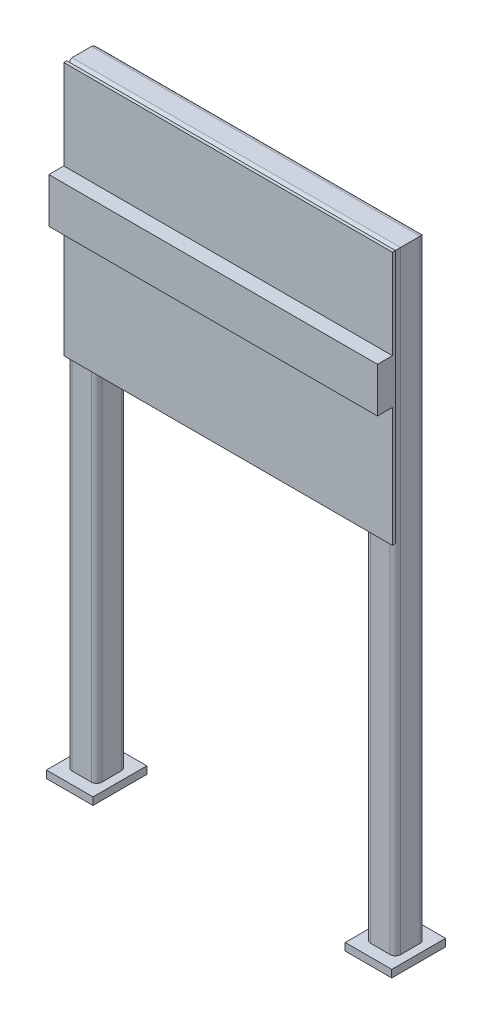
from build123d import *

# Parameters (mm, degrees)
GB_6728_1986_SQUARE_HOLLOW_SECTION_020_X_DEPTH = 415.142135624
GB_6728_1986_SQUARE_HOLLOW_SECTION_0_3_DEPTH   = 230.284271247
GB_6728_1986_SQUARE_HOLLOW_SECTION_0_5_DEPTH   = 415.142135624
GB_6728_1986_SQUARE_HOLLOW_SECTION_0_6_DEPTH   = 202
GB_6728_1986_SQUARE_HOLLOW_SECTION_0_8_DEPTH   = 202
SKETCH2_W                                      = 31.17404588
SKETCH2_H                                      = 36.03704403
BOSS_EXTRUDE1_DEPTH                            = 5
SKETCH3_W                                      = 220
SKETCH3_H                                      = 170
BOSS_EXTRUDE2_DEPTH                            = 2
SKETCH4_W                                      = 220
SKETCH4_H                                      = 30
BOSS_EXTRUDE3_DEPTH                            = 10


with BuildPart() as part:
    # Sketch1 → GB/6728-1986 square hollow section 020 X 20 X 1.75(1) (new body)
    with BuildSketch(Plane(origin=(-100, 0, 0), x_dir=(-1, 0, 0), z_dir=(0, 1, 0))):
        with BuildLine():
            Line((-6.5, -10), (6.5, -10))
            ThreePointArc((6.5, -10), (8.974873734, -8.974873734), (10, -6.5))
            Line((10, -6.5), (10, 6.5))
            ThreePointArc((10, 6.5), (8.974873734, 8.974873734), (6.5, 10))
            Line((6.5, 10), (-6.5, 10))
            ThreePointArc((-6.5, 10), (-8.974873734, 8.974873734), (-10, 6.5))
            Line((-10, 6.5), (-10, -6.5))
            ThreePointArc((-10, -6.5), (-8.974873734, -8.974873734), (-6.5, -10))
        make_face()
        with BuildLine():
            Line((-6.5, -8.25), (6.5, -8.25))
            ThreePointArc((6.5, -8.25), (7.737436867, -7.737436867), (8.25, -6.5))
            Line((8.25, -6.5), (8.25, 6.5))
            ThreePointArc((8.25, 6.5), (7.737436867, 7.737436867), (6.5, 8.25))
            Line((6.5, 8.25), (-6.5, 8.25))
            ThreePointArc((-6.5, 8.25), (-7.737436867, 7.737436867), (-8.25, 6.5))
            Line((-8.25, 6.5), (-8.25, -6.5))
            ThreePointArc((-8.25, -6.5), (-7.737436867, -7.737436867), (-6.5, -8.25))
        make_face(mode=Mode.SUBTRACT)
    extrude(amount=GB_6728_1986_SQUARE_HOLLOW_SECTION_020_X_DEPTH)

    # GB_6728-1986 square hollow section 0 2
    split(bisect_by=Plane(origin=(-100, 400, 0), x_dir=(0.707106781, -0.707106781, 0), z_dir=(-0.707106781, -0.707106781, 0)), keep=Keep.TOP)



with BuildPart() as body_2:
    # Sketch1 on segment 2 (carried to segment 2) → GB_6728-1986 square hollow section 0 3 (new body)
    with BuildSketch(Plane(origin=(-115.142135624, 400, 0), x_dir=(0, 1, 0), z_dir=(1, 0, 0))):
        with BuildLine():
            Line((-6.5, -10), (6.5, -10))
            ThreePointArc((6.5, -10), (8.974873734, -8.974873734), (10, -6.5))
            Line((10, -6.5), (10, 6.5))
            ThreePointArc((10, 6.5), (8.974873734, 8.974873734), (6.5, 10))
            Line((6.5, 10), (-6.5, 10))
            ThreePointArc((-6.5, 10), (-8.974873734, 8.974873734), (-10, 6.5))
            Line((-10, 6.5), (-10, -6.5))
            ThreePointArc((-10, -6.5), (-8.974873734, -8.974873734), (-6.5, -10))
        make_face()
        with BuildLine():
            Line((-6.5, -8.25), (6.5, -8.25))
            ThreePointArc((6.5, -8.25), (7.737436867, -7.737436867), (8.25, -6.5))
            Line((8.25, -6.5), (8.25, 6.5))
            ThreePointArc((8.25, 6.5), (7.737436867, 7.737436867), (6.5, 8.25))
            Line((6.5, 8.25), (-6.5, 8.25))
            ThreePointArc((-6.5, 8.25), (-7.737436867, 7.737436867), (-8.25, 6.5))
            Line((-8.25, 6.5), (-8.25, -6.5))
            ThreePointArc((-8.25, -6.5), (-7.737436867, -7.737436867), (-6.5, -8.25))
        make_face(mode=Mode.SUBTRACT)
    extrude(amount=GB_6728_1986_SQUARE_HOLLOW_SECTION_0_3_DEPTH)

    # GB_6728-1986 square hollow section 0 3 m
    split(bisect_by=Plane(origin=(-100, 400, 0), x_dir=(-0.707106781, 0.707106781, 0), z_dir=(0.707106781, 0.707106781, 0)), keep=Keep.TOP)

    # GB_6728-1986 square hollow section 0 4
    split(bisect_by=Plane(origin=(100, 400, 0), x_dir=(-0.707106781, -0.707106781, 0), z_dir=(-0.707106781, 0.707106781, 0)), keep=Keep.TOP)


with BuildPart() as body_3:
    # Sketch1 on segment 3 (carried to segment 3) → GB_6728-1986 square hollow section 0 5 (new body)
    with BuildSketch(Plane(origin=(100, 415.142135624, 0), x_dir=(1, 0, 0), z_dir=(0, -1, 0))):
        with BuildLine():
            Line((-6.5, -10), (6.5, -10))
            ThreePointArc((6.5, -10), (8.974873734, -8.974873734), (10, -6.5))
            Line((10, -6.5), (10, 6.5))
            ThreePointArc((10, 6.5), (8.974873734, 8.974873734), (6.5, 10))
            Line((6.5, 10), (-6.5, 10))
            ThreePointArc((-6.5, 10), (-8.974873734, 8.974873734), (-10, 6.5))
            Line((-10, 6.5), (-10, -6.5))
            ThreePointArc((-10, -6.5), (-8.974873734, -8.974873734), (-6.5, -10))
        make_face()
        with BuildLine():
            Line((-6.5, -8.25), (6.5, -8.25))
            ThreePointArc((6.5, -8.25), (7.737436867, -7.737436867), (8.25, -6.5))
            Line((8.25, -6.5), (8.25, 6.5))
            ThreePointArc((8.25, 6.5), (7.737436867, 7.737436867), (6.5, 8.25))
            Line((6.5, 8.25), (-6.5, 8.25))
            ThreePointArc((-6.5, 8.25), (-7.737436867, 7.737436867), (-8.25, 6.5))
            Line((-8.25, 6.5), (-8.25, -6.5))
            ThreePointArc((-8.25, -6.5), (-7.737436867, -7.737436867), (-6.5, -8.25))
        make_face(mode=Mode.SUBTRACT)
    extrude(amount=GB_6728_1986_SQUARE_HOLLOW_SECTION_0_5_DEPTH)

    # GB_6728-1986 square hollow section 0 5 m
    split(bisect_by=Plane(origin=(100, 400, 0), x_dir=(0.707106781, 0.707106781, 0), z_dir=(0.707106781, -0.707106781, 0)), keep=Keep.TOP)


with BuildPart() as body_4:
    # Sketch1 on segment 4 (carried to segment 4) → GB_6728-1986 square hollow section 0 6 (new body)
    with BuildSketch(Plane(origin=(-101, 330, 0), x_dir=(0, 1, 0), z_dir=(1, 0, 0))):
        with BuildLine():
            Line((-6.5, -10), (6.5, -10))
            ThreePointArc((6.5, -10), (8.974873734, -8.974873734), (10, -6.5))
            Line((10, -6.5), (10, 6.5))
            ThreePointArc((10, 6.5), (8.974873734, 8.974873734), (6.5, 10))
            Line((6.5, 10), (-6.5, 10))
            ThreePointArc((-6.5, 10), (-8.974873734, 8.974873734), (-10, 6.5))
            Line((-10, 6.5), (-10, -6.5))
            ThreePointArc((-10, -6.5), (-8.974873734, -8.974873734), (-6.5, -10))
        make_face()
        with BuildLine():
            Line((-6.5, -8.25), (6.5, -8.25))
            ThreePointArc((6.5, -8.25), (7.737436867, -7.737436867), (8.25, -6.5))
            Line((8.25, -6.5), (8.25, 6.5))
            ThreePointArc((8.25, 6.5), (7.737436867, 7.737436867), (6.5, 8.25))
            Line((6.5, 8.25), (-6.5, 8.25))
            ThreePointArc((-6.5, 8.25), (-7.737436867, 7.737436867), (-8.25, 6.5))
            Line((-8.25, 6.5), (-8.25, -6.5))
            ThreePointArc((-8.25, -6.5), (-7.737436867, -7.737436867), (-6.5, -8.25))
        make_face(mode=Mode.SUBTRACT)
    extrude(amount=GB_6728_1986_SQUARE_HOLLOW_SECTION_0_6_DEPTH)

    # GB_6728-1986 square hollow section 0 6 m
    split(bisect_by=Plane(origin=(-90, 330, 0), x_dir=(0, 1, 0), z_dir=(1, 0, 0)), keep=Keep.TOP)

    # GB_6728-1986 square hollow section 0 7
    split(bisect_by=Plane(origin=(90, 330, 0), x_dir=(0, -1, 0), z_dir=(-1, 0, 0)), keep=Keep.TOP)


with BuildPart() as body_5:
    # Sketch1 on segment 5 (carried to segment 5) → GB_6728-1986 square hollow section 0 8 (new body)
    with BuildSketch(Plane(origin=(-101, 250, 0), x_dir=(0, 1, 0), z_dir=(1, 0, 0))):
        with BuildLine():
            Line((-6.5, -10), (6.5, -10))
            ThreePointArc((6.5, -10), (8.974873734, -8.974873734), (10, -6.5))
            Line((10, -6.5), (10, 6.5))
            ThreePointArc((10, 6.5), (8.974873734, 8.974873734), (6.5, 10))
            Line((6.5, 10), (-6.5, 10))
            ThreePointArc((-6.5, 10), (-8.974873734, 8.974873734), (-10, 6.5))
            Line((-10, 6.5), (-10, -6.5))
            ThreePointArc((-10, -6.5), (-8.974873734, -8.974873734), (-6.5, -10))
        make_face()
        with BuildLine():
            Line((-6.5, -8.25), (6.5, -8.25))
            ThreePointArc((6.5, -8.25), (7.737436867, -7.737436867), (8.25, -6.5))
            Line((8.25, -6.5), (8.25, 6.5))
            ThreePointArc((8.25, 6.5), (7.737436867, 7.737436867), (6.5, 8.25))
            Line((6.5, 8.25), (-6.5, 8.25))
            ThreePointArc((-6.5, 8.25), (-7.737436867, 7.737436867), (-8.25, 6.5))
            Line((-8.25, 6.5), (-8.25, -6.5))
            ThreePointArc((-8.25, -6.5), (-7.737436867, -7.737436867), (-6.5, -8.25))
        make_face(mode=Mode.SUBTRACT)
    extrude(amount=GB_6728_1986_SQUARE_HOLLOW_SECTION_0_8_DEPTH)

    # GB_6728-1986 square hollow section 0 8 m
    split(bisect_by=Plane(origin=(-90, 250, 0), x_dir=(0, 1, 0), z_dir=(1, 0, 0)), keep=Keep.TOP)

    # GB_6728-1986 square hollow section 0 9
    split(bisect_by=Plane(origin=(90, 250, 0), x_dir=(0, -1, 0), z_dir=(-1, 0, 0)), keep=Keep.TOP)


with BuildPart() as part_1:
    add(part.part)

    add(body_3.part)  # Boss-Extrude1 merges body 3
    # Sketch2 → Boss-Extrude1 (add)
    with BuildSketch(Plane.XZ):
        with Locations((-100, 0)):
            Rectangle(SKETCH2_W, SKETCH2_H)
        with Locations((100, 0)):
            Rectangle(SKETCH2_W, SKETCH2_H)
    extrude(amount=BOSS_EXTRUDE1_DEPTH)


    add(body_2.part)  # Boss-Extrude2 merges body 2

    add(body_4.part)  # Boss-Extrude2 merges body 4

    add(body_5.part)  # Boss-Extrude2 merges body 5
    # Sketch3 → Boss-Extrude2 (add)
    with BuildSketch(Plane.XY.offset(10)):
        with Locations((0, 325)):
            Rectangle(SKETCH3_W, SKETCH3_H)
    extrude(amount=BOSS_EXTRUDE2_DEPTH)

    # Sketch4 → Boss-Extrude3 (add)
    with BuildSketch(Plane.XY.offset(12)):
        with Locations((0, 335)):
            Rectangle(SKETCH4_W, SKETCH4_H)
    extrude(amount=BOSS_EXTRUDE3_DEPTH)


solid = part_1.part
